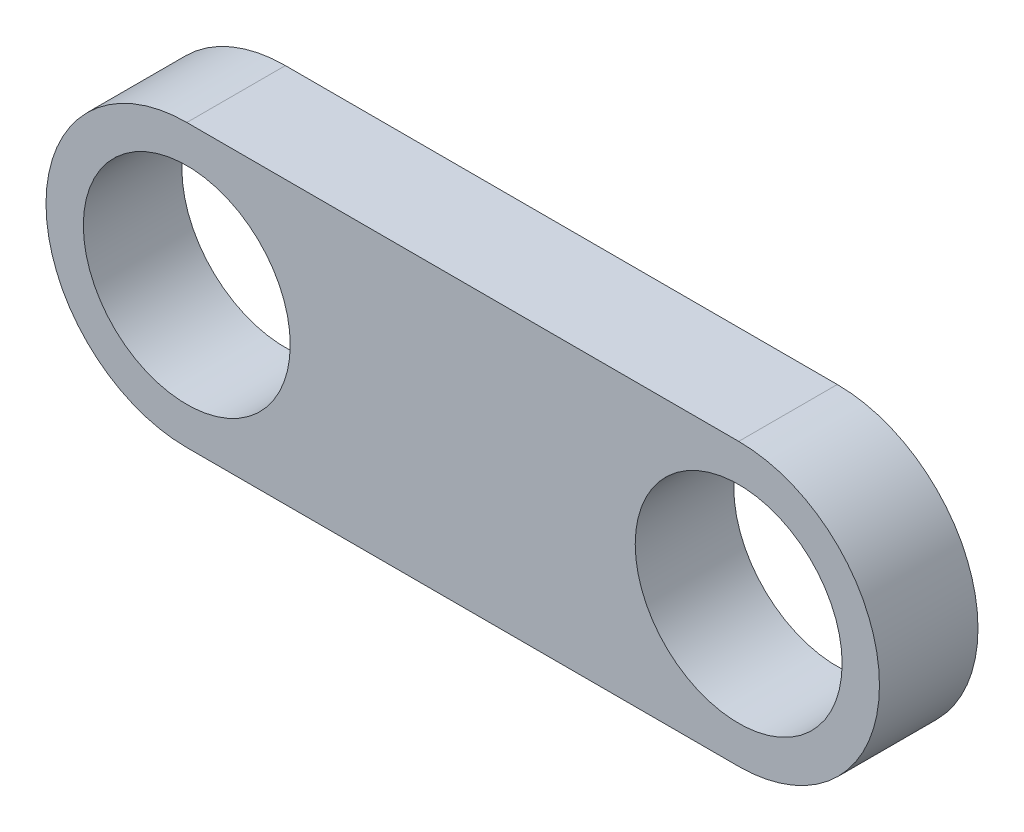
from build123d import *

# Parameters (mm, degrees)
BOSS_EXTRUDE1_DEPTH = 3.5
CUT_EXTRUDE1_REACH  = 34.643
SKETCH2_R           = 3.674588618


with BuildPart() as part:
    # Sketch1 → Boss-Extrude1 (new body)
    with BuildSketch(Plane.XY):
        with BuildLine():
            Line((7.466046977, 5.007712178), (27.067619065, 4.999999613))
            ThreePointArc((27.067619065, 4.999999613), (32.065651345, -0.001967333), (27.063684399, -4.999999613))
            Line((27.063684399, -4.999999613), (7.462112311, -4.992287048))
            ThreePointArc((7.462112311, -4.992287048), (2.464080031, 0.009679898), (7.466046977, 5.007712178))
        make_face()
    extrude(amount=BOSS_EXTRUDE1_DEPTH)

    # Sketch2 → Cut-Extrude1 (cut, up to next)
    with BuildSketch(Plane(origin=(0, 0, 0), x_dir=(-1, 0, 0), z_dir=(0, 0, -1)), mode=Mode.PRIVATE) as cut_extrude1_sk1:
        with Locations((-27.065651732, 0)):
            Circle(SKETCH2_R)
    cut_extrude1_tool1 = extrude(cut_extrude1_sk1.sketch, amount=-CUT_EXTRUDE1_REACH, mode=Mode.PRIVATE) & part.part
    # Sketch2 → Cut-Extrude1 (cut, up to next)
    with BuildSketch(Plane(origin=(0, 0, 0), x_dir=(-1, 0, 0), z_dir=(0, 0, -1)), mode=Mode.PRIVATE) as cut_extrude1_sk2:
        with Locations((-7.464079644, 0.007712565)):
            Circle(SKETCH2_R)
    cut_extrude1_tool2 = extrude(cut_extrude1_sk2.sketch, amount=-CUT_EXTRUDE1_REACH, mode=Mode.PRIVATE) & part.part
    add(cut_extrude1_tool1.solids().sort_by_distance((27.065652, 0, 0))[0], mode=Mode.SUBTRACT)
    add(cut_extrude1_tool2.solids().sort_by_distance((7.46408, 0.007713, 0))[0], mode=Mode.SUBTRACT)


solid = part.part
